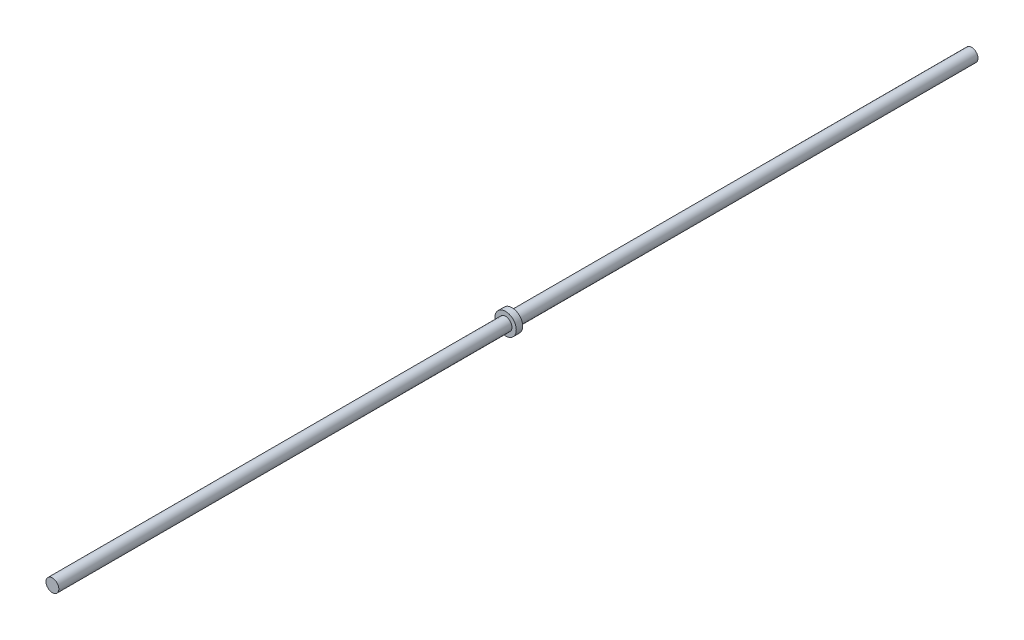
from build123d import *

# Parameters (mm, degrees)
SKETCH_1_W      = 3
SKETCH_1_H      = 430
EXTRUDE_START   = -215
SKETCH_3_R      = 5
EXTRUDE_1_DEPTH = 3


with BuildPart() as part:
    # 草图1 → 旋转1 (revolve)
    with BuildSketch(Plane(origin=(0, 0, 0), x_dir=(1, 0, 0), z_dir=(0, 1, 0))):
        with Locations((1.5, 215)):
            Rectangle(SKETCH_1_W, SKETCH_1_H)
    revolve(axis=Axis((0, 0, 0), (0, 0, -1)))

    # 草图3 → 凸台-拉伸1 (add)
    with BuildSketch(Plane.XY.offset(EXTRUDE_START)):
        Circle(SKETCH_3_R)
    extrude(amount=EXTRUDE_1_DEPTH)


solid = part.part
